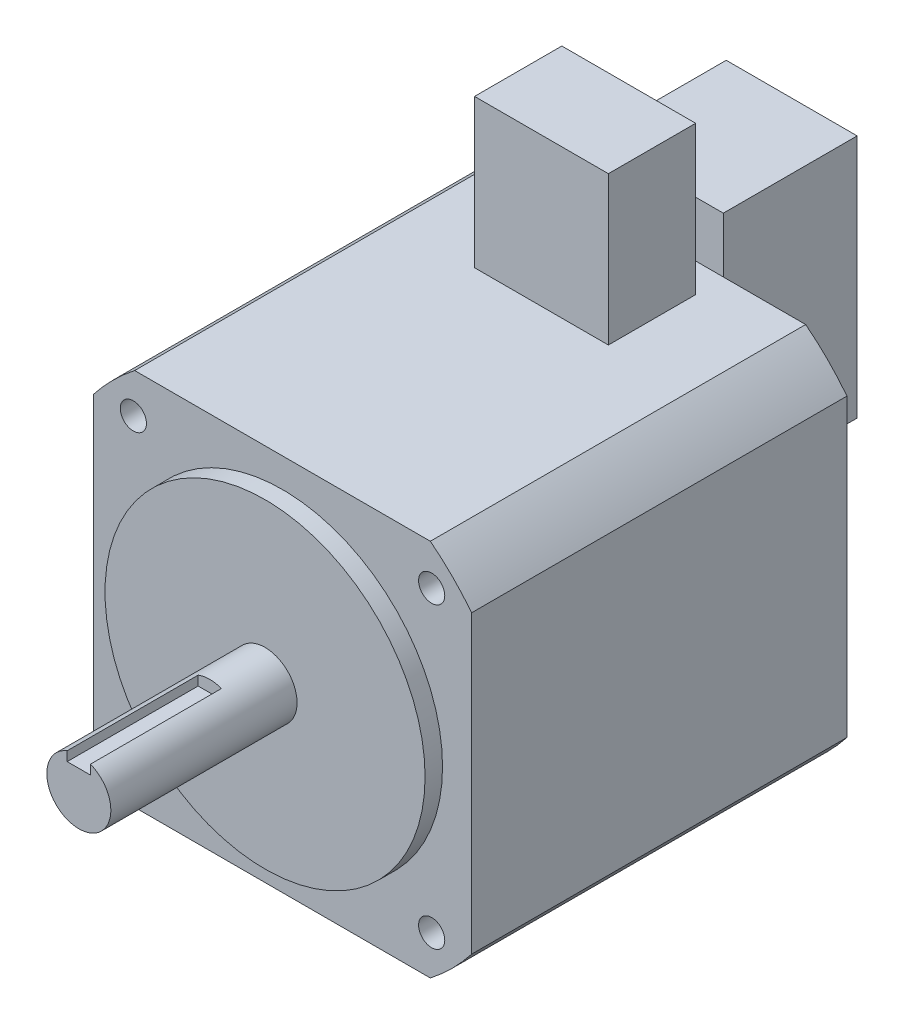
from build123d import *
from build123d.topology import SkipClean

# Parameters (mm, degrees)
SKETCH1_W           = 130
SKETCH1_H           = 130
BOSS_EXTRUDE1_DEPTH = 12
SKETCH2_R           = 55
BOSS_EXTRUDE2_DEPTH = 6
SKETCH3_R           = 11
BOSS_EXTRUDE3_DEPTH = 64
SKETCH4_OUTSIDE_W   = 172.262
SKETCH4_OUTSIDE_H   = 172.262
SKETCH4_OUTSIDE_R   = 82.5
CUT_EXTRUDE1_DEPTH  = 64
CIRPATTERN1_COUNT   = 4
BOSS_EXTRUDE4_DEPTH = 117
SKETCH8_W           = 45
SKETCH8_H           = 84
BOSS_EXTRUDE5_DEPTH = 46
SKETCH9_W           = 30
SKETCH9_H           = 51
BOSS_EXTRUDE6_DEPTH = 23
SKETCH10_W          = 8
SKETCH10_H          = 10
CUT_EXTRUDE2_DEPTH  = 45


with BuildPart() as part:
    # Sketch1 → Boss-Extrude1 (new body)
    with BuildSketch(Plane.XY):
        Rectangle(SKETCH1_W, SKETCH1_H)
    extrude(amount=BOSS_EXTRUDE1_DEPTH)

    # Sketch2 → Boss-Extrude2 (add)
    with BuildSketch(Plane.XY.offset(12)):
        Circle(SKETCH2_R)
    extrude(amount=BOSS_EXTRUDE2_DEPTH)

    # Sketch3 → Boss-Extrude3 (add)
    with BuildSketch(Plane.XY.offset(18)):
        Circle(SKETCH3_R)
    extrude(amount=BOSS_EXTRUDE3_DEPTH)

    # Sketch4 outside → Cut-Extrude1 (cut)
    with BuildSketch(Plane.XY.offset(12)):
        Rectangle(SKETCH4_OUTSIDE_W, SKETCH4_OUTSIDE_H)
        Circle(SKETCH4_OUTSIDE_R, mode=Mode.SUBTRACT)
    extrude(amount=-CUT_EXTRUDE1_DEPTH, mode=Mode.SUBTRACT)

    # Sketch5 → Ø9.0 (9) Diameter Hole1 (revolve, cut)
    with BuildSketch(Plane(origin=(-51.265241636, 51.265241636, 12), x_dir=(0, -1, 0), z_dir=(1, 0, 0))):
        Polygon((0, 0), (0, 402.703872786), (4.5, 400), (4.5, 0), align=None)
    f_9_0_9_diameter_hole1 = revolve(axis=Axis((-51.265241636, 51.265241636, 18.35), (0, 0, -1)), mode=Mode.SUBTRACT)

    # CirPattern1: Ø9.0 (9) Diameter Hole1 ×4 about axis
    cirpattern1_axis = Axis((0, 0, 0), (0, 0, 1))
    for i in range(1, CIRPATTERN1_COUNT):
        add(f_9_0_9_diameter_hole1.rotate(cirpattern1_axis, i * 360 / CIRPATTERN1_COUNT), mode=Mode.SUBTRACT)

    # Sketch7 → Boss-Extrude4 (add)
    with SkipClean():  # the faces are left unmerged after this step: merging them gives an invalid solid
        with BuildSketch(Plane(origin=(0, 0, 0), x_dir=(-1, 0, 0), z_dir=(0, 0, -1))):
            with BuildLine():
                Line((-65, 50.806003582), (-65, -50.806003582))
                ThreePointArc((-65, -50.806003582), (-58.336309448, -58.336309448), (-50.806003582, -65))
                Line((-50.806003582, -65), (50.806003582, -65))
                ThreePointArc((50.806003582, -65), (58.336309448, -58.336309448), (65, -50.806003582))
                Line((65, -50.806003582), (65, 50.806003582))
                ThreePointArc((65, 50.806003582), (58.336309448, 58.336309448), (50.806003582, 65))
                Line((50.806003582, 65), (-50.806003582, 65))
                ThreePointArc((-50.806003582, 65), (-58.336309448, 58.336309448), (-65, 50.806003582))
            make_face()
        extrude(amount=BOSS_EXTRUDE4_DEPTH)

    # Sketch8 → Boss-Extrude5 (add)
    with SkipClean():  # the faces are left unmerged after this step: merging them gives an invalid solid
        with BuildSketch(Plane(origin=(0, 0, -117), x_dir=(-1, 0, 0), z_dir=(0, 0, -1))):
            with Locations((0, 42)):
                Rectangle(SKETCH8_W, SKETCH8_H)
        extrude(amount=BOSS_EXTRUDE5_DEPTH)

    # Sketch9 → Boss-Extrude6 (add, symmetric)
    with SkipClean():  # the faces are left unmerged after this step: merging them gives an invalid solid
        with BuildSketch(Plane(origin=(0, 0, 0), x_dir=(0, 0, -1), z_dir=(1, 0, 0))):
            with Locations((92, 90.5)):
                Rectangle(SKETCH9_W, SKETCH9_H)
        extrude(amount=BOSS_EXTRUDE6_DEPTH, both=True)

    # Sketch10 → Cut-Extrude2 (cut)
    with SkipClean():  # the faces are left unmerged after this step: merging them gives an invalid solid
        with BuildSketch(Plane.XY.offset(82)):
            with Locations((0, 12)):
                Rectangle(SKETCH10_W, SKETCH10_H)
        extrude(amount=-CUT_EXTRUDE2_DEPTH, mode=Mode.SUBTRACT)


solid = part.part
